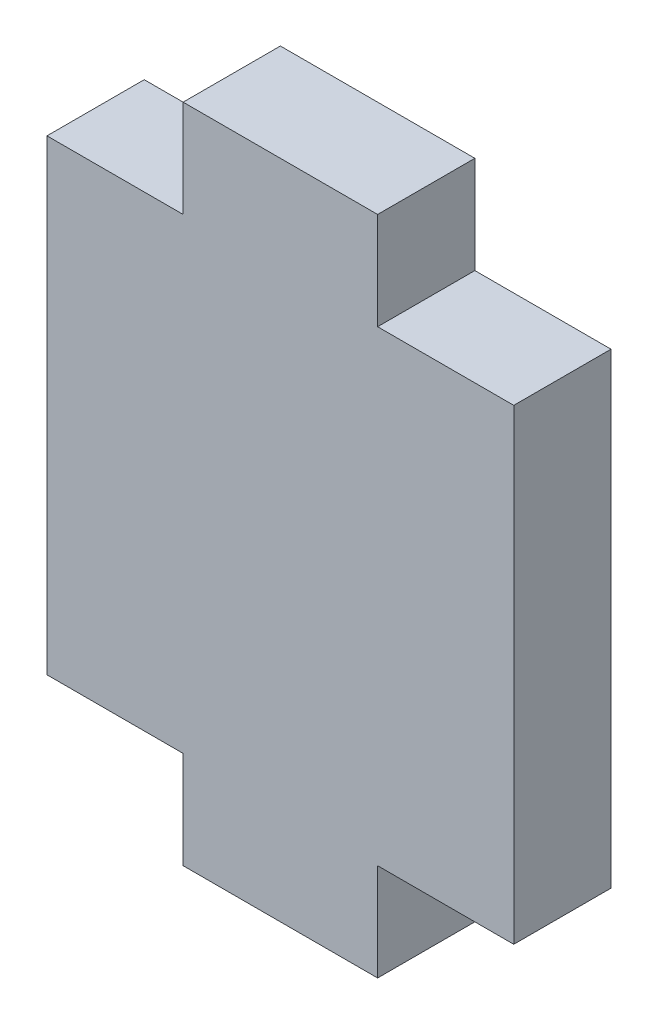
from build123d import *

# Parameters (mm, degrees)
SKETCH1_W           = 48
SKETCH1_H           = 68
BOSS_EXTRUDE1_DEPTH = 10
SKETCH2_W           = 28
SKETCH2_H           = 20
CUT_EXTRUDE1_DEPTH  = 10


with BuildPart() as part:
    # Sketch1 → Boss-Extrude1 (new body)
    with BuildSketch(Plane.XY):
        Rectangle(SKETCH1_W, SKETCH1_H)
    extrude(amount=BOSS_EXTRUDE1_DEPTH)

    # Sketch2 → Cut-Extrude1 (cut)
    with BuildSketch(Plane.XY.offset(10)):
        with Locations((-24, 34)):
            Rectangle(SKETCH2_W, SKETCH2_H)
        with Locations((24, 34)):
            Rectangle(SKETCH2_W, SKETCH2_H)
        with Locations((24, -34)):
            Rectangle(SKETCH2_W, SKETCH2_H)
        with Locations((-24, -34)):
            Rectangle(SKETCH2_W, SKETCH2_H)
    extrude(amount=-CUT_EXTRUDE1_DEPTH, mode=Mode.SUBTRACT)


solid = part.part
